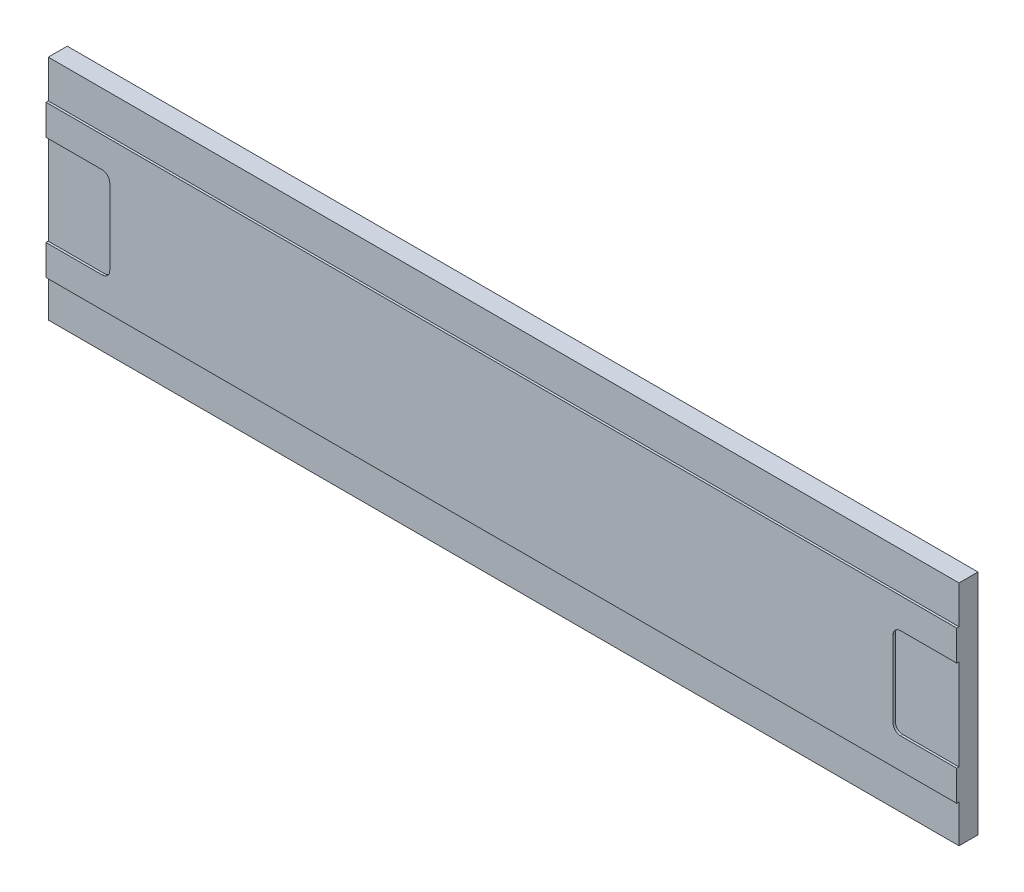
SolidWorks part; units mm, degrees
ref_plane "前视基准面" through (0, 0, 0) normal (0, 0, 1) x (1, 0, 0)
ref_plane "上视基准面" through (0, 0, 0) normal (0, 1, 0) x (1, 0, 0)
ref_plane "右视基准面" through (0, 0, 0) normal (1, 0, 0) x (0, 0, -1)
sketch "草图1" plane through (0, 0, 0) normal (0, 0, 1) x (1, 0, 0)
  line L0 (-300, 71.3806) -> (-300, 56.6194) construction
  line L1 (-300, -75) -> (300, -75)
  line L2 (-300, -75) -> (-300, 75)
  line L3 (-300, 75) -> (300, 75)
  line L4 (300, -75) -> (300, 75)
  line L5 (-300, -75) -> (300, 75) construction
  line L6 (-300, 75) -> (300, -75) construction
  point P0 (0, 0)
  dimension "D2" = 150
extrude "凸台-拉伸1" add sketch "草图1" along normal blind 14
sketch "草图2" plane through (0, 0, 14) normal (0, 0, 1) x (1, 0, 0)
  line L0 (300, -75) -> (300, 75) construction
  line L1 (-300, 75) -> (300, 75)
  line L2 (-300, 75) -> (-300, 50)
  line L3 (-300, 50) -> (300, 50)
  line L4 (300, 75) -> (300, 50)
  line L5 (-300, 75) -> (-300, -75) construction
  line L6 (-300, -75) -> (300, -75)
  line L7 (-300, -75) -> (-300, -50)
  line L8 (-300, -50) -> (300, -50)
  line L9 (300, -75) -> (300, -50)
  dimension "D1" = 25
  dimension "D2" = 25
extrude "切除-拉伸1" cut sketch "草图2" against normal blind 1.5
sketch "草图3" plane through (0, 0, 14) normal (0, 0, 1) x (1, 0, 0)
  line L0 (-300, 50) -> (-300, -50) construction
  line L1 (-300, -30) -> (-258, -30)
  line L2 (-300, -30) -> (-300, 30)
  line L3 (-300, 30) -> (-258, 30)
  line L4 (-258, -30) -> (-258, 30)
  line L5 (-300, -30) -> (-258, 30) construction
  line L6 (-300, 30) -> (-258, -30) construction
  line L7 (300, -50) -> (300, 50) construction
  line L8 (258, -30) -> (300, -30)
  line L9 (258, -30) -> (258, 30)
  line L10 (258, 30) -> (300, 30)
  line L11 (300, -30) -> (300, 30)
  line L12 (258, -30) -> (300, 30) construction
  line L13 (258, 30) -> (300, -30) construction
  point P0 (-279, 0)
  point P10 (279, 0)
  dimension "D1" = 60
  dimension "D2" = 42
  dimension "D3" = 42
extrude "切除-拉伸2" cut sketch "草图3" against normal blind 1.5
sketch "草图4" plane through (0, 0, 14) normal (0, 0, 1) x (1, 0, 0)
  line L0 (-258, 30) -> (-257, 30)
  line L1 (-257, 10) -> (-258, 10)
  line L2 (-258, -30) -> (-258, 30) construction
  line L3 (-258, 10) -> (-258, 30)
  line L4 (258, 30) -> (257, 30)
  line L5 (257, 10) -> (258, 10)
  line L6 (258, 30) -> (258, -30) construction
  line L7 (258, 10) -> (258, 30)
  line L8 (258, 0) -> (300, 0) construction
  line L9 (258, 30) -> (258, -30) construction
  line L10 (300, -30) -> (300, 30) construction
  line L11 (258, -10) -> (258, -30)
  line L12 (257, -10) -> (258, -10)
  line L13 (258, -30) -> (257, -30)
  line L14 (-258, -10) -> (-258, -30)
  line L15 (-257, -10) -> (-258, -10)
  line L16 (-258, -30) -> (-257, -30)
  arc A0 (-257, 30) -> (-257, 10) centre (-257, 20) cw
  arc A1 (257, 30) -> (257, 10) centre (257, 20) ccw
  arc A2 (257, -30) -> (257, -10) centre (257, -20) cw
  arc A3 (-257, -30) -> (-257, -10) centre (-257, -20) ccw
  dimension "D2" = 10
  dimension "D1" = 1
  dimension "D3" = 1
extrude "切除-拉伸3" [suppressed] cut sketch "草图4" against normal blind 1.5
fillet "圆角1" radius 5 4 edges at (258, -30, 13.25) (258, 30, 13.25) (-258, -30, 13.25) (-258, 30, 13.25)
